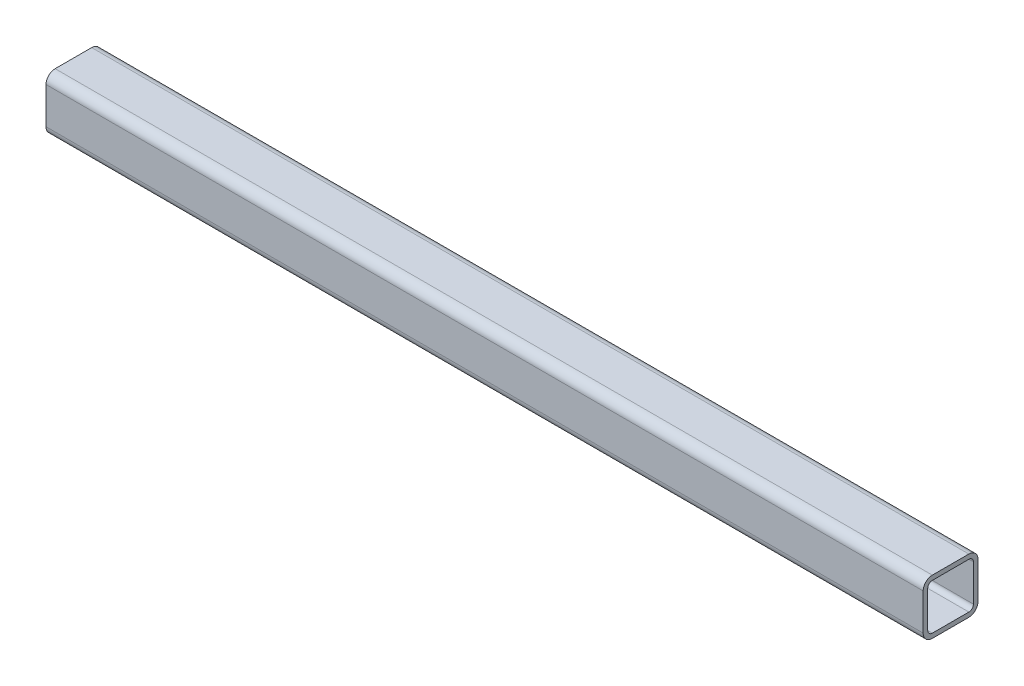
SolidWorks part; units mm, degrees
ref_plane "Front Plane" through (0, 0, 0) normal (0, 0, 1) x (1, 0, 0)
ref_plane "Top Plane" through (0, 0, 0) normal (0, 1, 0) x (1, 0, 0)
ref_plane "Right Plane" through (0, 0, 0) normal (1, 0, 0) x (0, 0, -1)
sketch "Sketch1" plane through (0, 0, 0) normal (0, 0, 1) x (1, 0, 0)
  line L0 (-240, 0) -> (240, 0)
  point P3 (0, 0)
  dimension "D1" = 480
other "Square tube 30 X 30 X 2.5"
ref_plane "Plane1" through (-240, 0, 0) normal (1, 0, 0) x (0, 1, 0)
sketch "Sketch16" plane through (-240, 0, 0) normal (1, 0, 0) x (0, 1, 0)
  line L0 (-10, -12.5) -> (10, -12.5)
  line L1 (-12.5, -10) -> (-12.5, 10)
  line L2 (10, 12.5) -> (-10, 12.5)
  line L3 (12.5, 10) -> (12.5, -10)
  line L4 (-10, -15) -> (10, -15)
  line L5 (-15, -10) -> (-15, 10)
  line L6 (10, 15) -> (-10, 15)
  line L7 (15, 10) -> (15, -10)
  arc A0 (15, 10) -> (10, 15) centre (10, 10) ccw
  arc A1 (10, -15) -> (15, -10) centre (10, -10) ccw
  arc A2 (-15, -10) -> (-10, -15) centre (-10, -10) ccw
  arc A3 (-10, 15) -> (-15, 10) centre (-10, 10) ccw
  arc A4 (-10, 12.5) -> (-12.5, 10) centre (-10, 10) ccw
  arc A5 (12.5, 10) -> (10, 12.5) centre (10, 10) ccw
  arc A6 (10, -12.5) -> (12.5, -10) centre (10, -10) ccw
  arc A7 (-12.5, -10) -> (-10, -12.5) centre (-10, -10) ccw
  point P0 (-15, 0)
  point P1 (15, 0)
  point P2 (0, 15)
  point P3 (0, -15)
  point P4 (0, 0)
  point P5 (-15, -15)
  point P6 (15, -15)
  point P7 (15, 15)
  point P8 (-15, 15)
  point P33 (0, 0)
  dimension "D1" = 5
  dimension "Thickness" = 2.5
  dimension "V_leg" = 30
